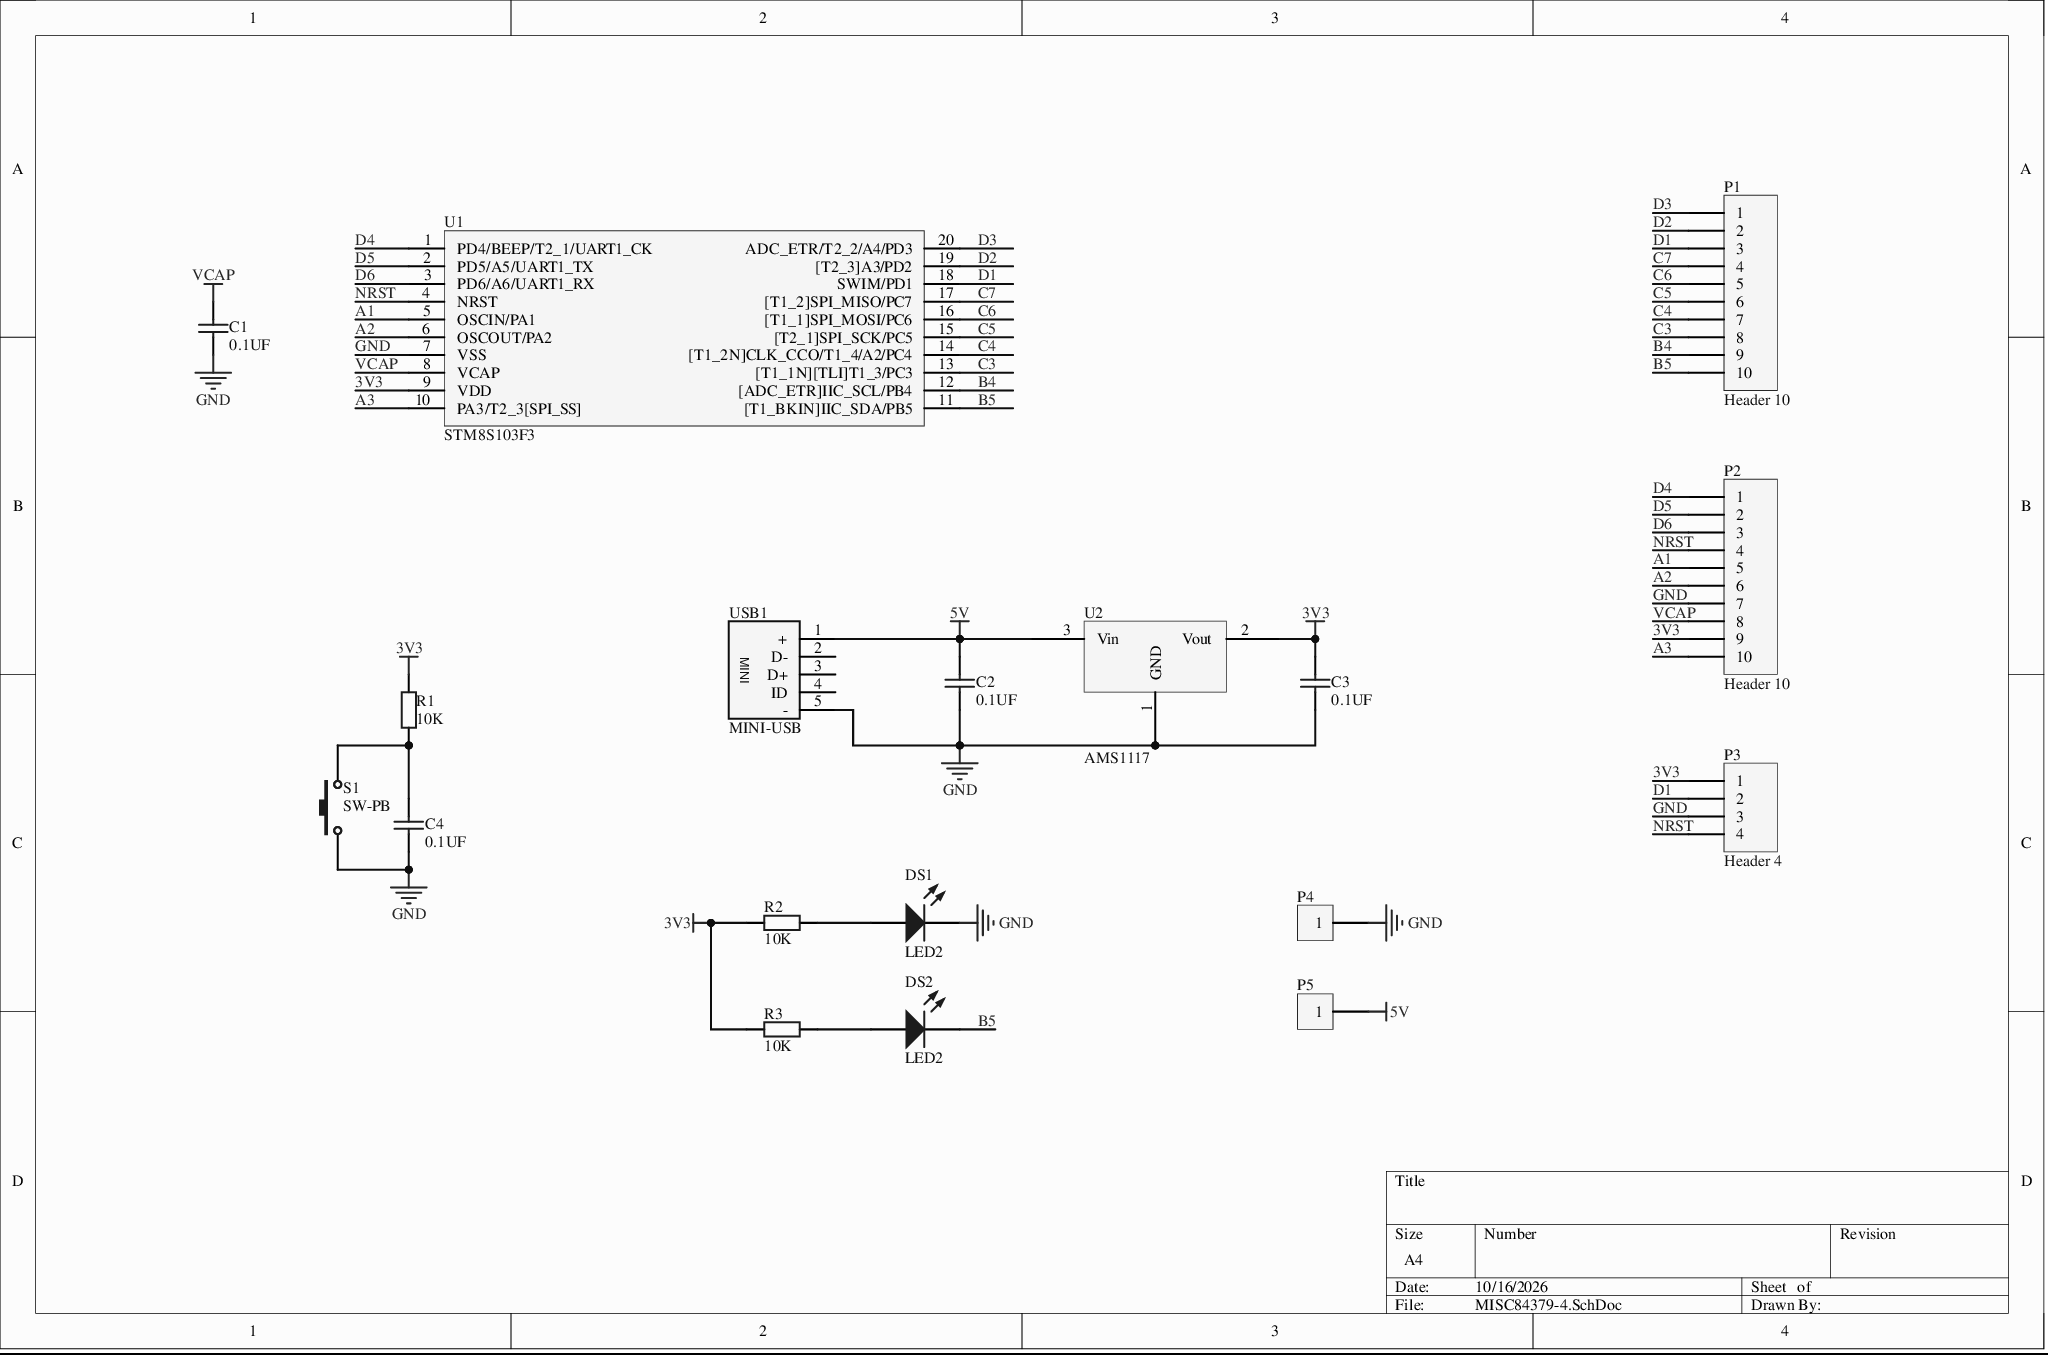
[diagram p0: MISC84379-4.SchDoc]
# Altium project MISC84379-5.PrjPcb
1 sheet, 18 parts. Net scope: global (net labels, ports and power ports of the same name join across sheets).
Board file: MISC84379.PcbDoc

## Sheet MISC84379-4.SchDoc
size A4

### Parts
C1  0.1UF  [C1206]
C2  0.1UF  [C1206]
C3  0.1UF  [C1206]
C4  0.1UF  [C1206]
DS1  LED2  [my0603LED]
DS2  LED2  [my0603LED]
P1  Header 10  [HDR1X10]
P2  Header 10  [HDR1X10]
P3  Header 4  [HDR1X4]
P4  HDR1X1  [HDR1X1]  (value not drawn)
P5  HDR1X1  [HDR1X1]  (value not drawn)
R1  value 10K  [my0603]  (hidden comment: Res2)
R2  value 10K  [my0603]  (hidden comment: Res2)
R3  value 10K  [my0603]  (hidden comment: Res2)
S1  SW-PB  [SW_PB2_A1]
U1  STM8S103F3  [SOP-20]
U2  AMS1117  [SOT223]
USB1  MINI-USB  [USB-MINI-A]

### Nets
3V3: C3.2 P2.9 P3.1 R1.2 R2.2 R3.2 U1.9(VDD) U2.2(Vout)
5V: C2.2 P5.1 U2.3(Vin) USB1.1(+)
GND: C1.1 C2.1 C3.1 C4.1 DS1.2(K) P2.7 P3.3 P4.1 S1.1 U1.7(VSS) U2.1(GND) USB1.5(-)
VCAP: C1.2 P2.8 U1.8(VCAP)
A1: P2.5 U1.5(OSCIN/PA1)
A2: P2.6 U1.6(OSCOUT/PA2)
A3: P2.10 U1.10(PA3/T2_3[SPI_SS])
B4: P1.9 U1.12([ADC_ETR]IIC_SCL/PB4)
B5: DS2.2(K) P1.10 U1.11([T1_BKIN]IIC_SDA/PB5)
C3: P1.8 U1.13([T1_1N][TLI]T1_3/PC3)
C4: P1.7 U1.14([T1_2N]CLK_CCO/T1_4/A2/PC4)
C5: P1.6 U1.15([T2_1]SPI_SCK/PC5)
C6: P1.5 U1.16([T1_1]SPI_MOSI/PC6)
C7: P1.4 U1.17([T1_2]SPI_MISO/PC7)
D1: P1.3 P3.2 U1.18(SWIM/PD1)
D2: P1.2 U1.19([T2_3]A3/PD2)
D3: P1.1 U1.20(ADC_ETR/T2_2/A4/PD3)
D4: P2.1 U1.1(PD4/BEEP/T2_1/UART1_CK)
D5: P2.2 U1.2(PD5/A5/UART1_TX)
D6: P2.3 U1.3(PD6/A6/UART1_RX)
NRST: P2.4 P3.4 U1.4(NRST)
NetC4_2: C4.2 R1.1 S1.2
NetDS1_1: DS1.1(A) R2.1
NetDS2_1: DS2.1(A) R3.1

Not connected (* = marked no-connect by the designer): USB1 2(D-) 3(D+) 4(ID)

### Library data of the parts
C1-C4 = Cap Semi: Capacitor (Semiconductor SIM Model); Published: 8-Jun-2000; LatestRevisionDate: 29-May-2009; LatestRevisionNote: IPC-7351 Footprint Added.; PackageReference: C1206; PackageDescription: Chip Capacitor; Publisher: Altium Limited
DS1 DS2 = LED2: Typical RED, GREEN, YELLOW, AMBER GaAs LED; Published: 8-Jun-2000; LatestRevisionDate: 17-Jul-2002; LatestRevisionNote: Re-released for DXP Platform.; PackageDocument: Feb-2002; PackageReference: 3.2X1.6X1.1; Publisher: Altium Limited
P1 P2 = Header 10: Header, 10-Pin; LatestRevisionDate: 17-Jul-2002; LatestRevisionNote: Re-released for DXP Platform.; Publisher: Altium Limited
P3 = Header 4: Header, 4-Pin; LatestRevisionDate: 17-Jul-2002; LatestRevisionNote: Re-released for DXP Platform.; Publisher: Altium Limited
R1-R3 = Res2: Resistor; Published: 8-Jun-2000; LatestRevisionDate: 17-Jul-2002; LatestRevisionNote: Re-released for DXP Platform.; PackageReference: AXIAL-0.4; PackageDescription: Axial Device, Thru-Hole; 2 Leads; 0.4 in Pin Spacing; Publisher: Altium Limited
S1 = SW-PB: Switch; Published: 24-Mar-1999; LatestRevisionDate: 17-Jul-2002; LatestRevisionNote: Re-released for DXP Platform.; Publisher: Altium Limited
U2 = AMS1117: Three-terminal regulator IC